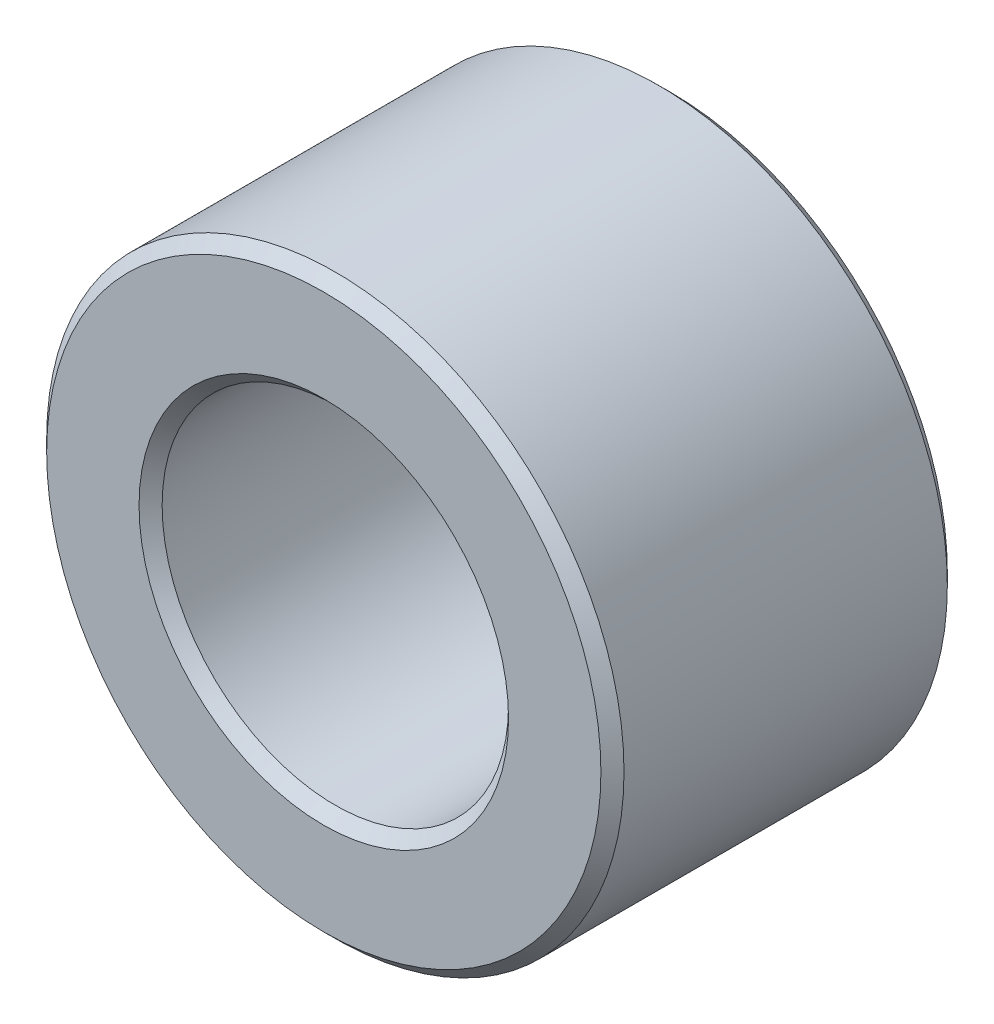
from build123d import *

# Parameters (mm, degrees)
SKETCH1_R           = 25
SKETCH1_R_2         = 15
BOSS_EXTRUDE1_DEPTH = 30
CHAMFER1_SIZE       = 1


with BuildPart() as part:
    # Sketch1 → Boss-Extrude1 (new body)
    with BuildSketch(Plane.XY):
        Circle(SKETCH1_R)
        Circle(SKETCH1_R_2, mode=Mode.SUBTRACT)
    extrude(amount=BOSS_EXTRUDE1_DEPTH)

    # Chamfer1
    chamfer1_edges = [part.edges().sort_by_distance(p)[0] for p in [
        (-25, 0, 0),
        (-25, 0, 30),
        (-15, 0, 0),
        (-15, 0, 30),
    ]]
    chamfer(chamfer1_edges, length=CHAMFER1_SIZE)


solid = part.part
